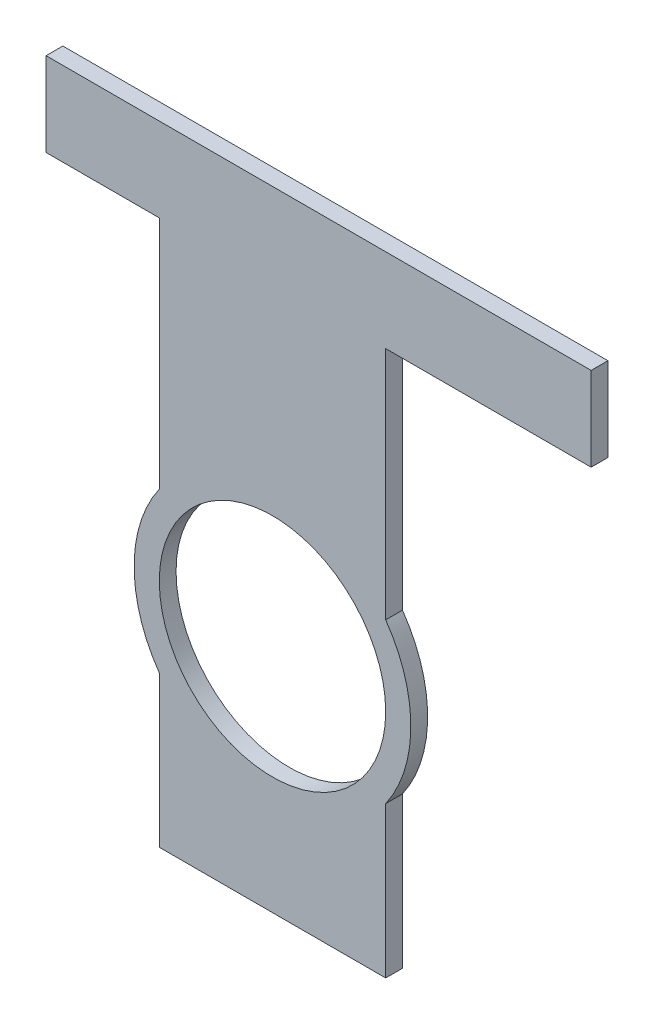
from build123d import *

# Parameters (mm, degrees)
SKETCH1_R           = 135
BOSS_EXTRUDE2_DEPTH = 20
SKETCH5_W           = 270
SKETCH5_H           = 200
CUT_EXTRUDE1_DEPTH  = 20
SKETCH6_W           = 245
SKETCH6_H           = 100
SKETCH6_W_2         = 135
BOSS_EXTRUDE3_DEPTH = 20


with BuildPart() as part:
    # Sketch1 → Boss-Extrude2 (new body)
    with BuildSketch(Plane.XY):
        with BuildLine():
            Line((-135, 475), (-135, 94.868329805))
            ThreePointArc((-135, 94.868329805), (-165, 0), (-135, -94.868329805))
            Line((-135, -94.868329805), (-135, -475))
            Line((-135, -475), (135, -475))
            Line((135, -475), (135, -94.868329805))
            ThreePointArc((135, -94.868329805), (165, 0), (135, 94.868329805))
            Line((135, 94.868329805), (135, 475))
            Line((135, 475), (-135, 475))
        make_face()
        Circle(SKETCH1_R, mode=Mode.SUBTRACT)
    extrude(amount=BOSS_EXTRUDE2_DEPTH)

    # Sketch5 → Cut-Extrude1 (cut)
    with BuildSketch(Plane.XY.offset(20)):
        with Locations((0, -375)):
            Rectangle(SKETCH5_W, SKETCH5_H)
    extrude(amount=-CUT_EXTRUDE1_DEPTH, mode=Mode.SUBTRACT)

    # Sketch6 → Boss-Extrude3 (add)
    with BuildSketch(Plane(origin=(0, 0, 0), x_dir=(-1, 0, 0), z_dir=(0, 0, -1))):
        with Locations((-257.5, 425)):
            Rectangle(SKETCH6_W, SKETCH6_H)
        with Locations((202.5, 425)):
            Rectangle(SKETCH6_W_2, SKETCH6_H)
    extrude(amount=-BOSS_EXTRUDE3_DEPTH)


solid = part.part
